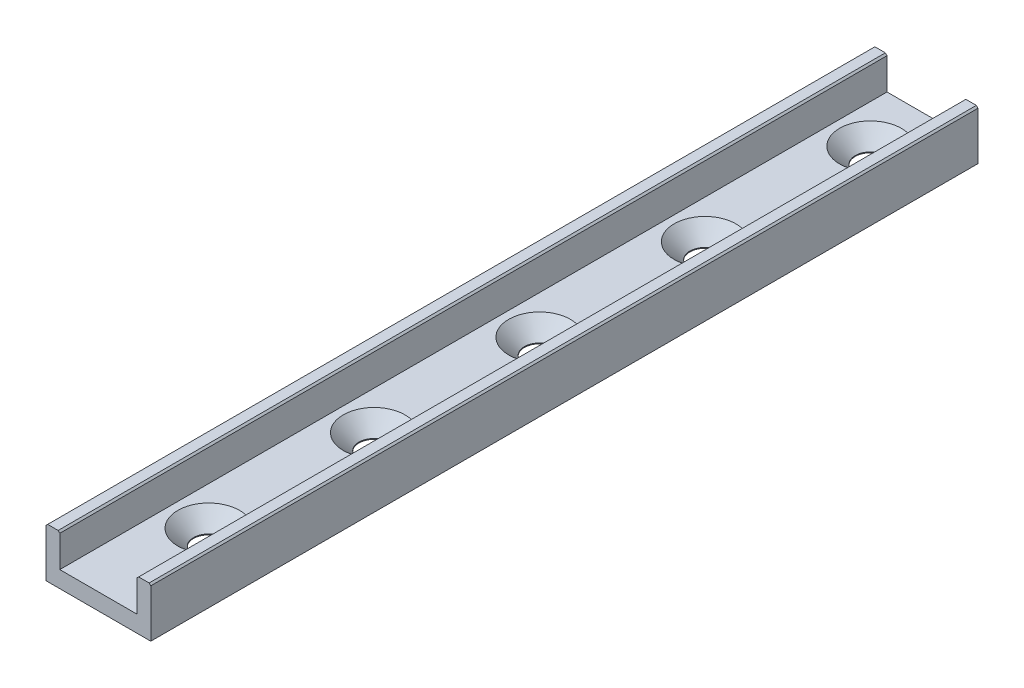
from build123d import *

# Parameters (mm, degrees)
BOSS_EXTRUDE1_DEPTH                          = 150
HOLE_SIZE_PER_PHILLIPS_SLOTTED_COUNT_2_COUNT = 2
HOLE_SIZE_PER_PHILLIPS_SLOTTED_COUNT_2_PITCH = 30
LPATTERN1_COUNT                              = 4
LPATTERN1_PITCH                              = 30
CHAMFER1_SIZE                                = 0.3


with BuildPart() as part:
    # Sketch1 → Boss-Extrude1 (new body)
    with BuildSketch(Plane.XY):
        Polygon((-7, 4.5), (-7, -1.5), (7, -1.5), (7, 4.5), (9.5, 4.5), (9.5, -4.5), (-9.5, -4.5), (-9.5, 4.5), align=None)
    extrude(amount=BOSS_EXTRUDE1_DEPTH)

    # Sketch5 → Hole size per Phillips slotted countersunk wood screw type 1 (revolve, cut)
    with BuildSketch(Plane(origin=(0, -1.5, 10), x_dir=(0, 0, 1), z_dir=(1, 0, 0))):
        Polygon((0, 0), (0, 3), (2.75, 3), (2.75, 2.85), (5.6, 0), align=None)
    hole_size_per_phillips_slotted_countersu = revolve(axis=Axis((0, 4.85, 10), (0, -1, 0)), mode=Mode.SUBTRACT)

    # Hole size per Phillips slotted count 2: Hole size per Phillips slotted countersunk wood screw type 1 ×2
    with Locations(*[(0, 0, i * HOLE_SIZE_PER_PHILLIPS_SLOTTED_COUNT_2_PITCH) for i in range(1, HOLE_SIZE_PER_PHILLIPS_SLOTTED_COUNT_2_COUNT)]):
        add(hole_size_per_phillips_slotted_countersu, mode=Mode.SUBTRACT)

    # LPattern1: Hole size per Phillips slotted countersunk wood screw type 1 ×4
    with Locations(*[(0, 0, i * LPATTERN1_PITCH) for i in range(1, LPATTERN1_COUNT)]):
        add(hole_size_per_phillips_slotted_countersu, mode=Mode.SUBTRACT)

    # LPattern1 copy 1 sketch → LPattern1 copy 1 (revolve, cut)
    with BuildSketch(Plane(origin=(0, -1.5, 70), x_dir=(0, 0, 1), z_dir=(1, 0, 0))):
        Polygon((0, 0), (0, 3), (2.75, 3), (2.75, 2.85), (5.6, 0), align=None)
    revolve(axis=Axis((0, 4.85, 70), (0, -1, 0)), mode=Mode.SUBTRACT)

    # LPattern1 copy 2 sketch → LPattern1 copy 2 (revolve, cut)
    with BuildSketch(Plane(origin=(0, -1.5, 100), x_dir=(0, 0, 1), z_dir=(1, 0, 0))):
        Polygon((0, 0), (0, 3), (2.75, 3), (2.75, 2.85), (5.6, 0), align=None)
    revolve(axis=Axis((0, 4.85, 100), (0, -1, 0)), mode=Mode.SUBTRACT)

    # LPattern1 copy 3 sketch → LPattern1 copy 3 (revolve, cut)
    with BuildSketch(Plane(origin=(0, -1.5, 130), x_dir=(0, 0, 1), z_dir=(1, 0, 0))):
        Polygon((0, 0), (0, 3), (2.75, 3), (2.75, 2.85), (5.6, 0), align=None)
    revolve(axis=Axis((0, 4.85, 130), (0, -1, 0)), mode=Mode.SUBTRACT)

    # Chamfer1
    chamfer1_edges = [part.edges().sort_by_distance(p)[0] for p in [
        (9.5, 4.5, 75),
        (-9.5, 4.5, 75),
        (-7, 4.5, 75),
        (7, 4.5, 75),
    ]]
    chamfer(chamfer1_edges, length=CHAMFER1_SIZE)


solid = part.part
